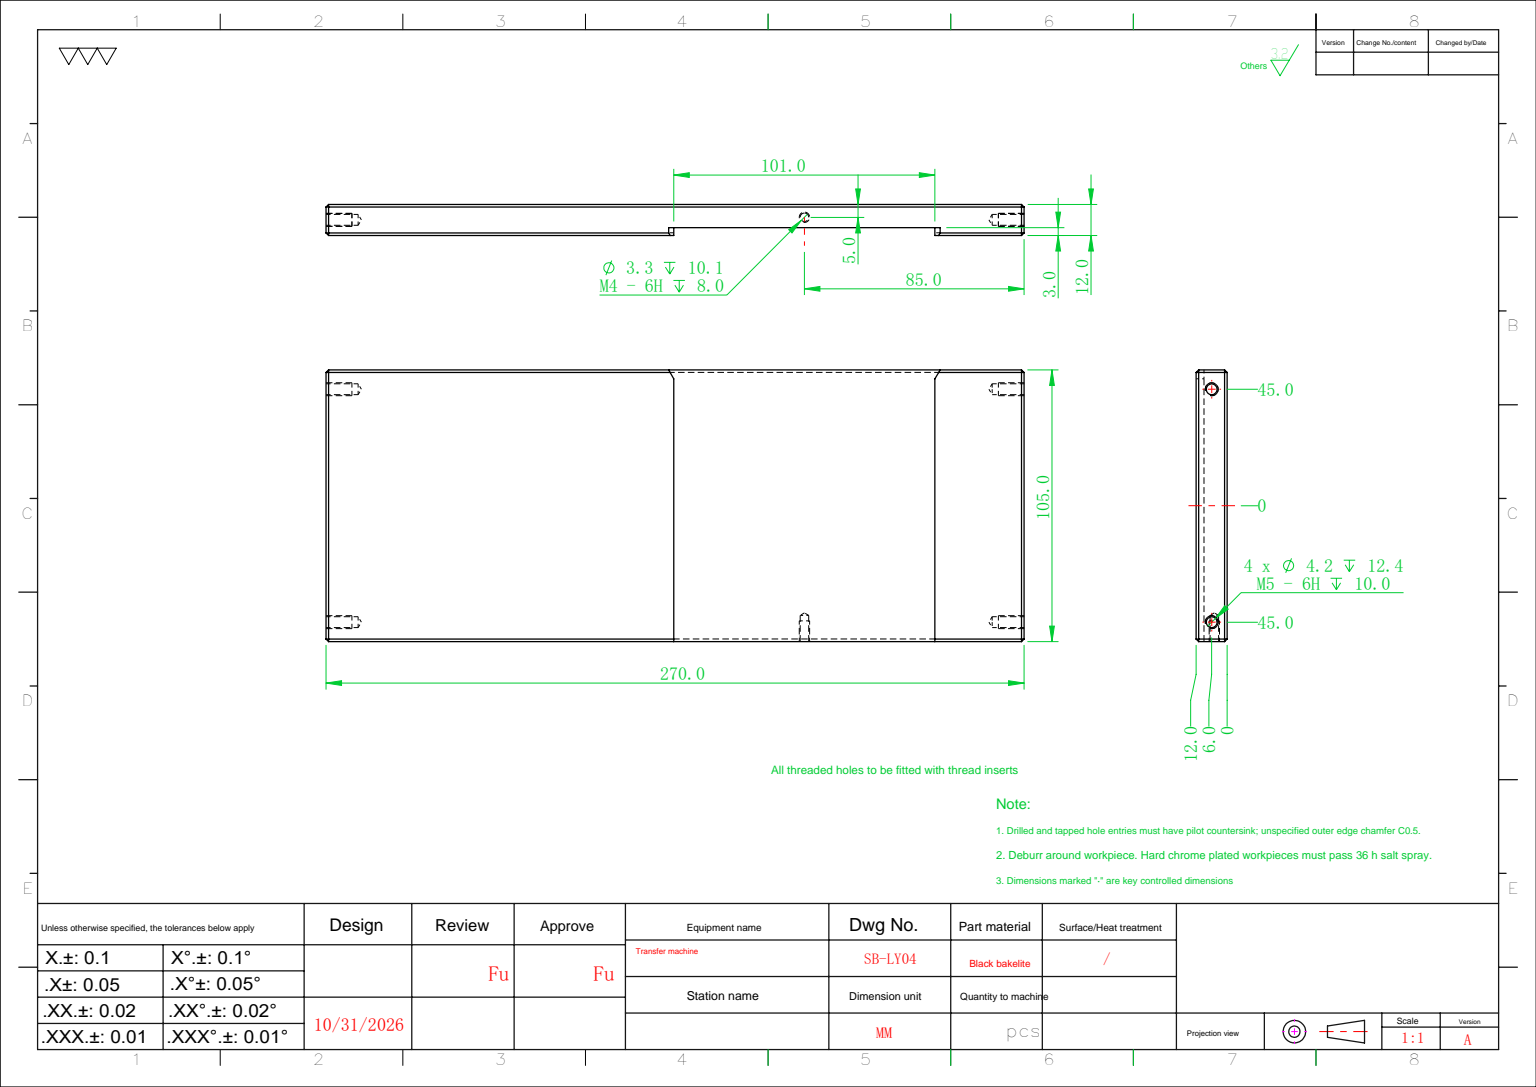
from build123d import *

# Parameters (mm, degrees)
SKETCH_1_W                  = 105
SKETCH_1_H                  = 270
EXTRUDE_1_DEPTH             = 12
SKETCH_2_W                  = 3
SKETCH_2_H                  = 101
CUT_EXTRUDE_1_DEPTH         = 172.446784747
HOLE_WIZARD_M5_1_AT_2_COUNT = 2
HOLE_WIZARD_M5_1_AT_2_PITCH = 90
CHAMFER_1_SIZE              = 1
CHAMFER_2_SIZE              = 2
CHAMFER_2_SIZE2             = 3.464101615
HOLE_WIZARD_M4_1_D          = 3.3
HOLE_WIZARD_M4_1_DEPTH      = 10.1
HOLE_WIZARD_M4_1_TIP        = 0.991420021


with BuildPart() as part:
    # 草图1 → 凸台-拉伸1 (new body)
    with BuildSketch(Plane.XY):
        Rectangle(SKETCH_1_W, SKETCH_1_H)
    extrude(amount=EXTRUDE_1_DEPTH)

    # 草图2 → 切除-拉伸1 (cut, through all)
    with BuildSketch(Plane(origin=(52.5, 0, 0), x_dir=(0, 0, -1), z_dir=(1, 0, 0))):
        with Locations((-10.5, 50)):
            Rectangle(SKETCH_2_W, SKETCH_2_H)
    extrude(amount=-CUT_EXTRUDE_1_DEPTH, mode=Mode.SUBTRACT)

    # 草图4 → M5 螺纹孔1 (revolve, cut)
    with BuildSketch(Plane(origin=(-45, -135, 6), x_dir=(0, 0, -1), z_dir=(1, 0, 0))):
        Polygon((0, 0), (0, 13.6618073), (2.1, 12.4), (2.1, 0), align=None)
    hole_wizard_m5_1 = revolve(axis=Axis((-45, -141.35, 6), (0, 1, 0)), mode=Mode.SUBTRACT)

    # M5 螺纹孔1 at 2: M5 螺纹孔1 ×2
    with Locations(*[(i * HOLE_WIZARD_M5_1_AT_2_PITCH, 0, 0) for i in range(1, HOLE_WIZARD_M5_1_AT_2_COUNT)]):
        add(hole_wizard_m5_1, mode=Mode.SUBTRACT)

    # 镜向1: M5 螺纹孔1 across plane
    add(hole_wizard_m5_1.mirror(Plane.ZX), mode=Mode.SUBTRACT)

    # 镜向1 copy 1 sketch → 镜向1 copy 1 (revolve, cut)
    with BuildSketch(Plane(origin=(45, 135, 6), x_dir=(0, 0, -1), z_dir=(1, 0, 0))):
        Polygon((0, 0), (0, -13.6618073), (2.1, -12.4), (2.1, 0), align=None)
    revolve(axis=Axis((45, 141.35, 6), (0, 1, 0)), mode=Mode.SUBTRACT)

    # 倒角1
    chamfer_1_edges = [part.edges().sort_by_distance(p)[0] for p in [
        (-52.5, 117.75, 12),
        (0, -135, 12),
        (52.5, 117.75, 12),
        (-52.5, -67.75, 12),
        (52.5, -67.75, 12),
        (0, -135, 0),
        (-52.5, 0, 0),
        (0, 135, 0),
        (52.5, 0, 0),
        (0, 135, 12),
        (52.5, -135, 6),
        (-52.5, -135, 6),
        (-52.5, 135, 6),
        (52.5, 135, 6),
    ]]
    chamfer(chamfer_1_edges, length=CHAMFER_1_SIZE)

    # 倒角2
    chamfer_2_edges = [part.edges().sort_by_distance(p)[0] for p in [
        (-52.5, -0.5, 10),
        (-52.5, 100.5, 10),
    ]]
    chamfer_2_side = [part.faces().sort_by_distance(p)[0] for p in [
        (-52.5, -4.075867635, 5.673930589),
    ]]
    chamfer(chamfer_2_edges, length=CHAMFER_2_SIZE, length2=CHAMFER_2_SIZE2, reference=chamfer_2_side[0])

    # M4 螺纹孔1
    with Locations(Plane(origin=(52.5, 0, 0), x_dir=(0, 0, -1), z_dir=(1, 0, 0))):
        with Locations((-5, 50)):
            Hole(HOLE_WIZARD_M4_1_D / 2, depth=HOLE_WIZARD_M4_1_DEPTH)
            with Locations((0, 0, -(HOLE_WIZARD_M4_1_DEPTH + HOLE_WIZARD_M4_1_TIP / 2))):  # 118° drill point
                Cone(0, HOLE_WIZARD_M4_1_D / 2, HOLE_WIZARD_M4_1_TIP, mode=Mode.SUBTRACT)


solid = part.part
